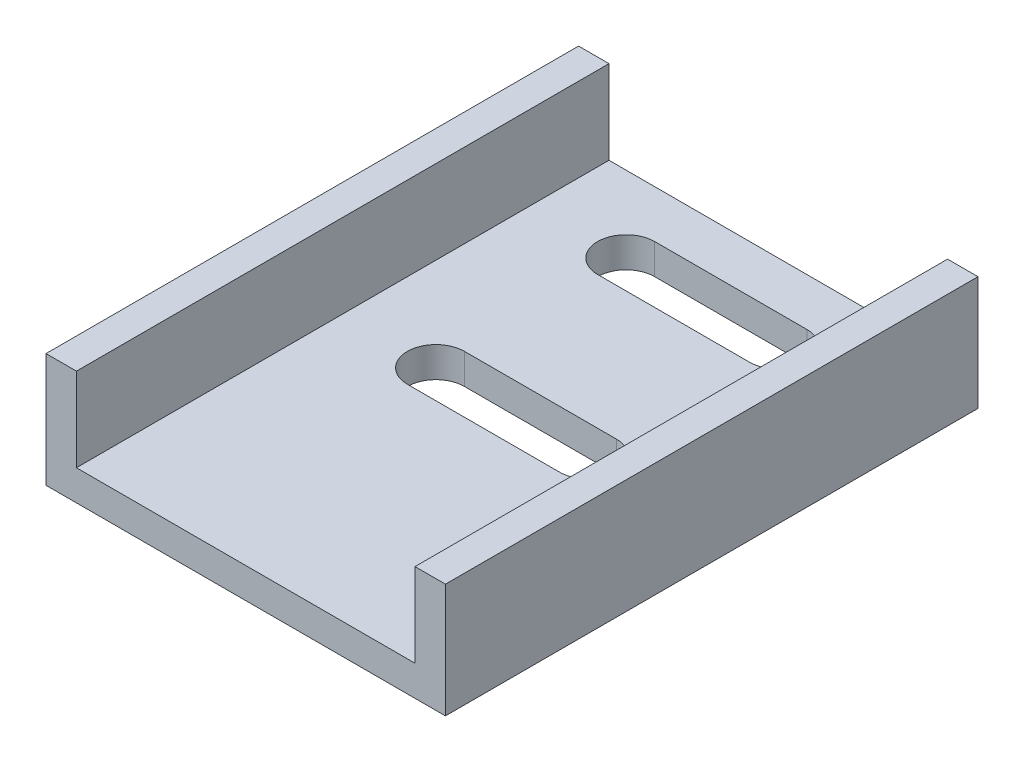
from build123d import *

# Parameters (mm, degrees)
EXTRUDE_1_DEPTH     = 140
CUT_EXTRUDE_1_DEPTH = 140


with BuildPart() as part:
    # 草图1 → 凸台-拉伸1 (new body)
    with BuildSketch(Plane.XY):
        Polygon((0, 0), (105, 0), (105, 30), (97, 30), (97, 8), (8, 8), (8, 30), (0, 30), align=None)
    extrude(amount=EXTRUDE_1_DEPTH)

    # 草图2 → 切除-拉伸1 (cut)
    with BuildSketch(Plane.XZ):
        with BuildLine():
            Line((52.5, 70), (52.5, 62.5))
            Line((52.5, 62.5), (72.5, 62.5))
            ThreePointArc((72.5, 62.5), (80, 70), (72.5, 77.5))
            Line((72.5, 77.5), (52.5, 77.5))
            Line((52.5, 77.5), (52.5, 70))
        make_face()
        with BuildLine():
            Line((32.5, 62.5), (52.5, 62.5))
            Line((52.5, 62.5), (52.5, 70))
            Line((52.5, 70), (52.5, 77.5))
            Line((52.5, 77.5), (32.5, 77.5))
            ThreePointArc((32.5, 77.5), (25, 70), (32.5, 62.5))
        make_face()
        with BuildLine():
            Line((32.5, 12.5), (52.5, 12.5))
            Line((52.5, 12.5), (52.5, 20))
            Line((52.5, 20), (52.5, 27.5))
            Line((52.5, 27.5), (32.5, 27.5))
            ThreePointArc((32.5, 27.5), (25, 20), (32.5, 12.5))
        make_face()
        with BuildLine():
            Line((52.5, 20), (52.5, 12.5))
            Line((52.5, 12.5), (72.5, 12.5))
            ThreePointArc((72.5, 12.5), (80, 20), (72.5, 27.5))
            Line((72.5, 27.5), (52.5, 27.5))
            Line((52.5, 27.5), (52.5, 20))
        make_face()
    extrude(amount=-CUT_EXTRUDE_1_DEPTH, mode=Mode.SUBTRACT)


solid = part.part
